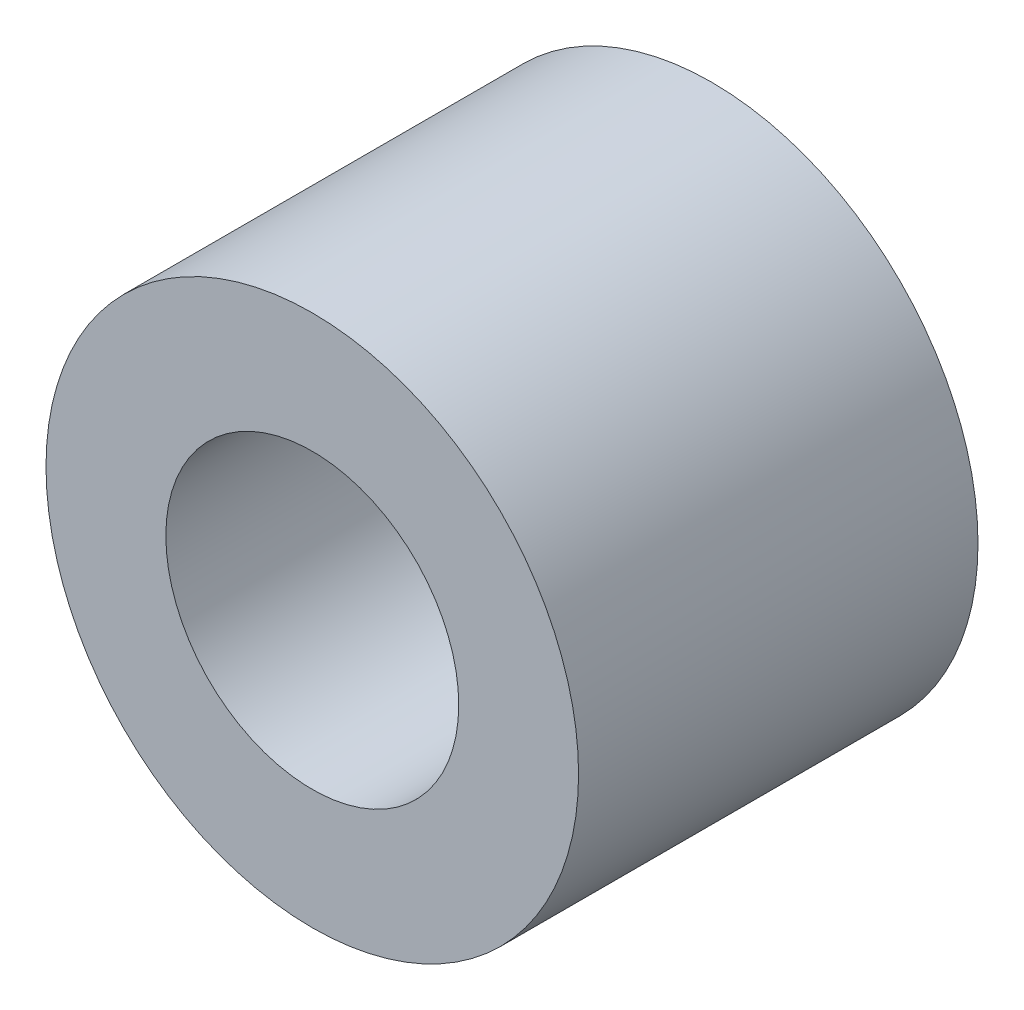
from build123d import *

# Parameters (mm, degrees)
SKETCH_1_R                = 10
EXTRUDE_1_DEPTH           = 15
HOLE_WIZARD_1_D           = 6.6
HOLE_WIZARD_1_CBORE_D     = 11
HOLE_WIZARD_1_CBORE_DEPTH = 8


with BuildPart() as part:
    # 草图1 → 凸台-拉伸1 (new body)
    with BuildSketch(Plane.XY):
        Circle(SKETCH_1_R)
    extrude(amount=EXTRUDE_1_DEPTH)

    # 打孔尺寸(%根据)内六角圆柱头螺钉的类型1 (through all)
    with Locations(Plane.XY.offset(15)):
        with Locations((0, 0)):
            CounterBoreHole(HOLE_WIZARD_1_D / 2, HOLE_WIZARD_1_CBORE_D / 2, HOLE_WIZARD_1_CBORE_DEPTH)


solid = part.part
